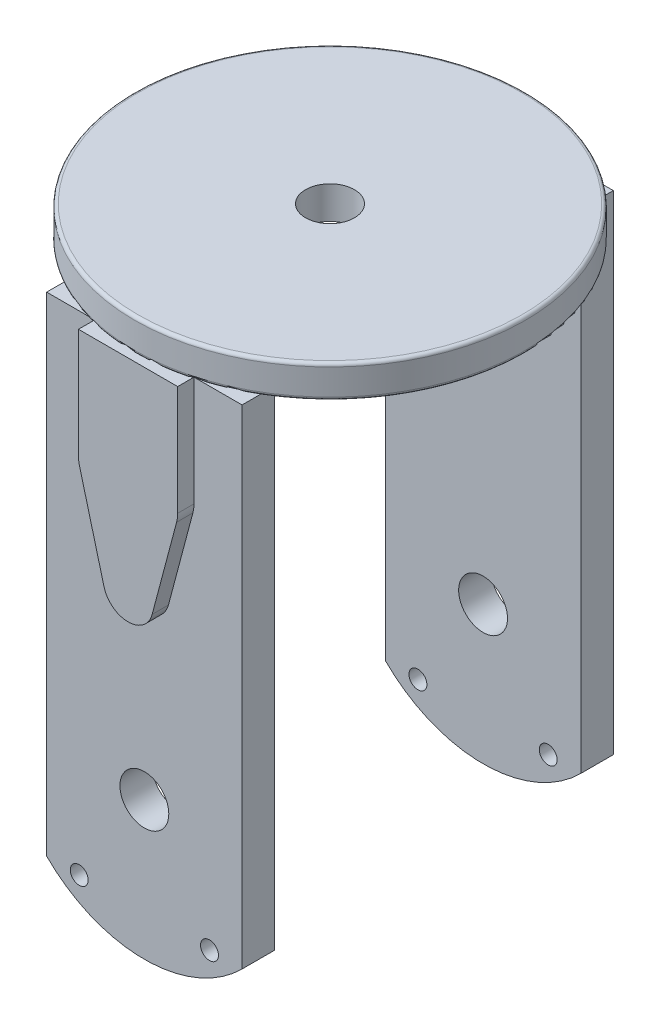
from build123d import *

# Parameters (mm, degrees)
SKETCH1_R           = 60
BOSS_EXTRUDE1_DEPTH = 10
FILLET2_R           = 1
SKETCH5_R           = 7.5
CUT_EXTRUDE2_DEPTH  = 86.440037535
SKETCH2_R           = 7.5
BOSS_EXTRUDE2_DEPTH = 10
BOSS_EXTRUDE4_DEPTH = 5


with BuildPart() as part:
    # Sketch1 → Boss-Extrude1 (new body)
    with BuildSketch(Plane(origin=(0, 0, 0), x_dir=(1, 0, 0), z_dir=(0, 1, 0))):
        with Locations(Location((0, 0, 0), (0, 0, 270))):
            Circle(SKETCH1_R)
    extrude(amount=BOSS_EXTRUDE1_DEPTH)

    # Fillet2
    fillet2_edges = [part.edges().sort_by_distance(p)[0] for p in [
        (0, 0, -60),
        (0, 10, -60),
    ]]
    fillet(fillet2_edges, radius=FILLET2_R)

    # Sketch5 → Cut-Extrude2 (cut, through all)
    with BuildSketch(Plane(origin=(0, 10, 0), x_dir=(1, 0, 0), z_dir=(0, 1, 0))):
        with Locations(Location((0, 0, 0), (0, 0, 270))):
            Circle(SKETCH5_R)
    cut_extrude2 = extrude(amount=-CUT_EXTRUDE2_DEPTH, mode=Mode.SUBTRACT)

    # Sketch2 → Boss-Extrude2 (add)
    with BuildSketch(Plane.XY.offset(47)):
        with BuildLine():
            Line((30, 0), (-30, 0))
            Line((-30, 0), (-30, -150))
            ThreePointArc((-30, -150), (0, -162.426406871), (30, -150))
            Line((30, -150), (30, 0))
        make_face()
        with Locations((0, -120)):
            Circle(SKETCH2_R, mode=Mode.SUBTRACT)
    boss_extrude2 = extrude(amount=BOSS_EXTRUDE2_DEPTH)

    # Sketch7 → Boss-Extrude4 (add)
    with BuildSketch(Plane.XY.offset(57)):
        with BuildLine():
            Line((-15.231546212, 0), (15.231546212, 0))
            Line((15.231546212, 0), (15.231546212, -33.694506244))
            ThreePointArc((15.231546212, -33.694506244), (15.147404529, -34.989015356), (14.896395444, -36.261740032))
            Line((14.896395444, -36.261740032), (7.393947913, -64.506158047))
            ThreePointArc((7.393947913, -64.506158047), (0, -70.192484331), (-7.393947913, -64.506158047))
            Line((-7.393947913, -64.506158047), (-14.896395444, -36.261740032))
            ThreePointArc((-14.896395444, -36.261740032), (-15.147404529, -34.989015356), (-15.231546212, -33.694506244))
            Line((-15.231546212, -33.694506244), (-15.231546212, 0))
        make_face()
    boss_extrude4 = extrude(amount=BOSS_EXTRUDE4_DEPTH)

    # Mirror2: Cut-Extrude2, Boss-Extrude2, Boss-Extrude4 across plane
    add(cut_extrude2.mirror(Plane.XY), mode=Mode.SUBTRACT)
    add(boss_extrude2.mirror(Plane.XY))
    add(boss_extrude4.mirror(Plane.XY))

    # Sketch10 → CBORE for M5 Hexagon head bolts-Full thread-grade C1 (revolve, cut)
    with BuildSketch(Plane(origin=(20, -150, -60), x_dir=(0, 1, 0), z_dir=(1, 0, 0))):
        Polygon((0, 0), (0, 122), (2.75, 122), (2.75, 0.5), (5.5, 0.5), (5.5, 0.025), (5.525, 0), align=None)
    cbore_for_m5_hexagon_head_bolts_full_thr = revolve(axis=Axis((20, -150, -66.35), (0, 0, 1)), mode=Mode.SUBTRACT)

    # Mirror3: CBORE for M5 Hexagon head bolts-Full thread-grade C1 across plane
    add(cbore_for_m5_hexagon_head_bolts_full_thr.mirror(Plane.ZY), mode=Mode.SUBTRACT)


solid = part.part
